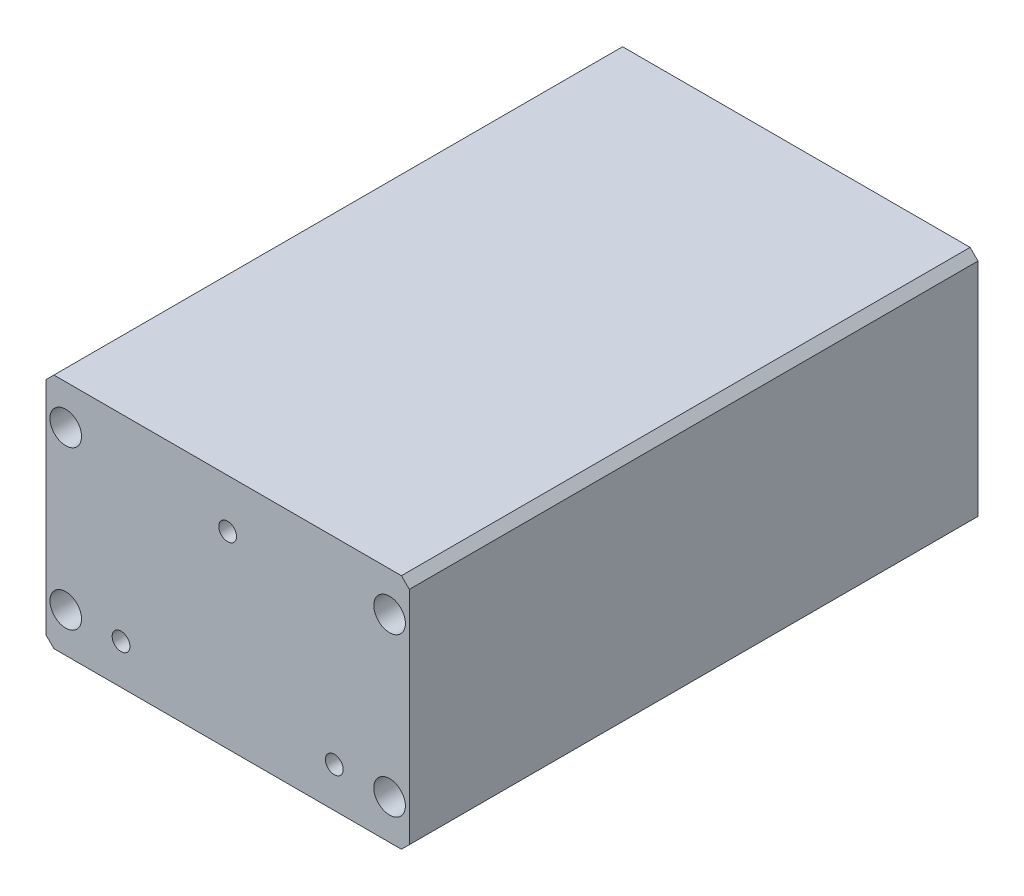
from build123d import *

# Parameters (mm, degrees)
SKETCH_1_W                   = 92
SKETCH_1_H                   = 60
EXTRUDE_1_DEPTH              = 144
HOLE_WIZARD_M4_1_D           = 4.5
HOLE_WIZARD_M4_1_CBORE_D     = 8
HOLE_WIZARD_M4_1_CBORE_DEPTH = 35
CHAMFER_1_SIZE               = 2
HOLE_WIZARD_M4_2_D           = 4.5
HOLE_WIZARD_M4_2_CBORE_D     = 8
HOLE_WIZARD_M4_2_CBORE_DEPTH = 37


with BuildPart() as part:
    # 草图1 → 凸台-拉伸1 (new body)
    with BuildSketch(Plane.XY):
        Rectangle(SKETCH_1_W, SKETCH_1_H)
    extrude(amount=EXTRUDE_1_DEPTH)

    # M4 六角凹头螺钉的柱形沉头孔1 (through all)
    with Locations(Plane.XY.offset(144)):
        with Locations((-41, 20), (-41, -20), (41, 20), (41, -20)):
            CounterBoreHole(HOLE_WIZARD_M4_1_D / 2, HOLE_WIZARD_M4_1_CBORE_D / 2, HOLE_WIZARD_M4_1_CBORE_DEPTH)

    # 倒角1
    chamfer_1_edges = [part.edges().sort_by_distance(p)[0] for p in [
        (46, -30, 72),
        (-46, -30, 72),
        (-46, 30, 72),
        (46, 30, 72),
    ]]
    chamfer(chamfer_1_edges, length=CHAMFER_1_SIZE)

    # M4 六角凹头螺钉的柱形沉头孔2 (through all)
    with Locations(Plane(origin=(0, 0, 0), x_dir=(-1, 0, 0), z_dir=(0, 0, -1))):
        with Locations((0, 17.7), (-27, -19.9), (27, -19.9)):
            CounterBoreHole(HOLE_WIZARD_M4_2_D / 2, HOLE_WIZARD_M4_2_CBORE_D / 2, HOLE_WIZARD_M4_2_CBORE_DEPTH)


solid = part.part
